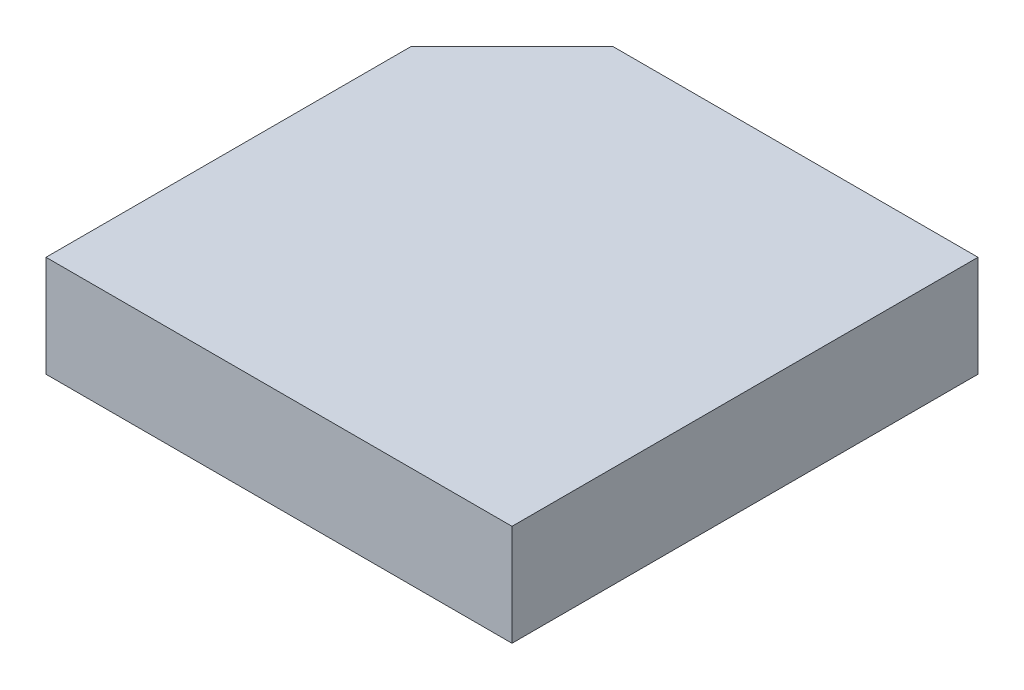
from build123d import *

# Parameters (mm, degrees)
EXTRUDE_1_DEPTH = 25


with BuildPart() as part:
    # 草图1 → 凸台-拉伸1 (new body)
    with BuildSketch(Plane(origin=(0, 0, 0), x_dir=(1, 0, 0), z_dir=(0, 1, 0))):
        Polygon((-115, 90), (-90, 115), (0, 115), (0, 0), (-115, 0), align=None)
    extrude(amount=EXTRUDE_1_DEPTH)


solid = part.part
